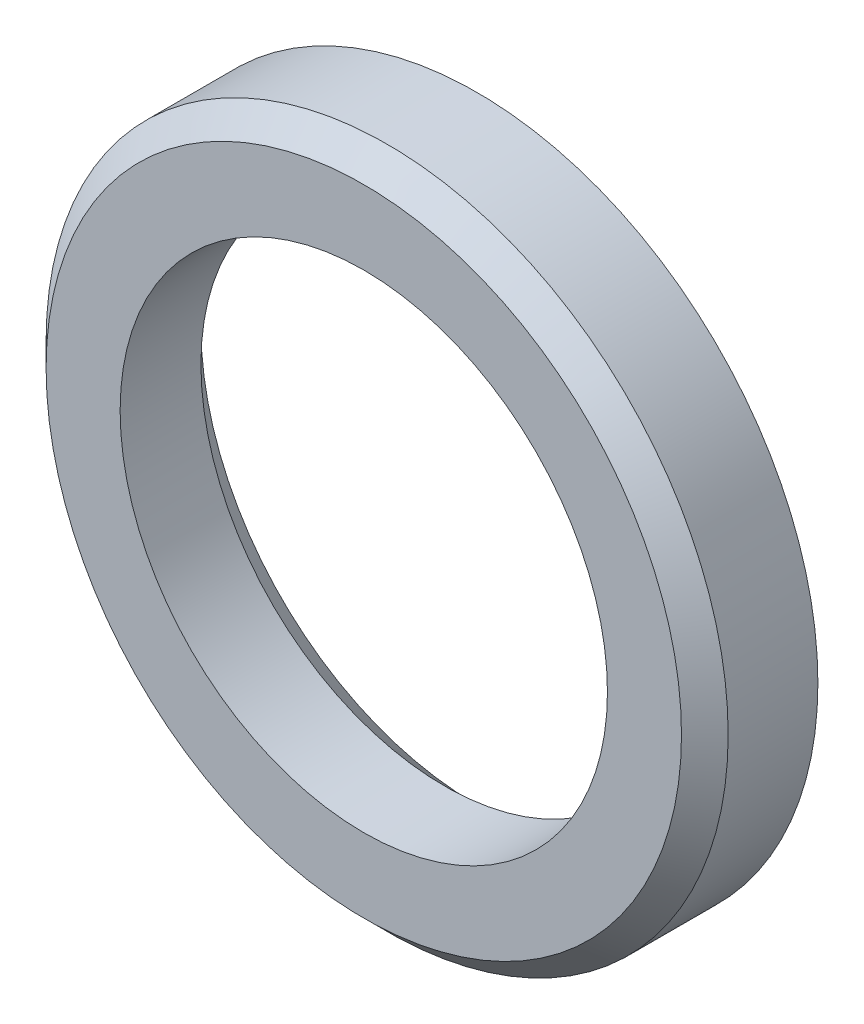
from build123d import *

# Parameters (mm, degrees)
SKETCH_1_R      = 19
SKETCH_1_R_2    = 13.575
EXTRUDE_1_DEPTH = 6.3
CHAMFER_1_SIZE  = 1.3
CHAMFER_2_SIZE  = 1.8


with BuildPart() as part:
    # 草图1 → 凸台-拉伸1 (new body)
    with BuildSketch(Plane.XY):
        Circle(SKETCH_1_R)
        Circle(SKETCH_1_R_2, mode=Mode.SUBTRACT)
    extrude(amount=EXTRUDE_1_DEPTH)

    # 倒角1
    chamfer_1_edges = [part.edges().sort_by_distance(p)[0] for p in [
        (-19, 0, 6.3),
    ]]
    chamfer(chamfer_1_edges, length=CHAMFER_1_SIZE)

    # 倒角2
    chamfer_2_edges = [part.edges().sort_by_distance(p)[0] for p in [
        (-13.575, 0, 0),
    ]]
    chamfer(chamfer_2_edges, length=CHAMFER_2_SIZE)


solid = part.part
